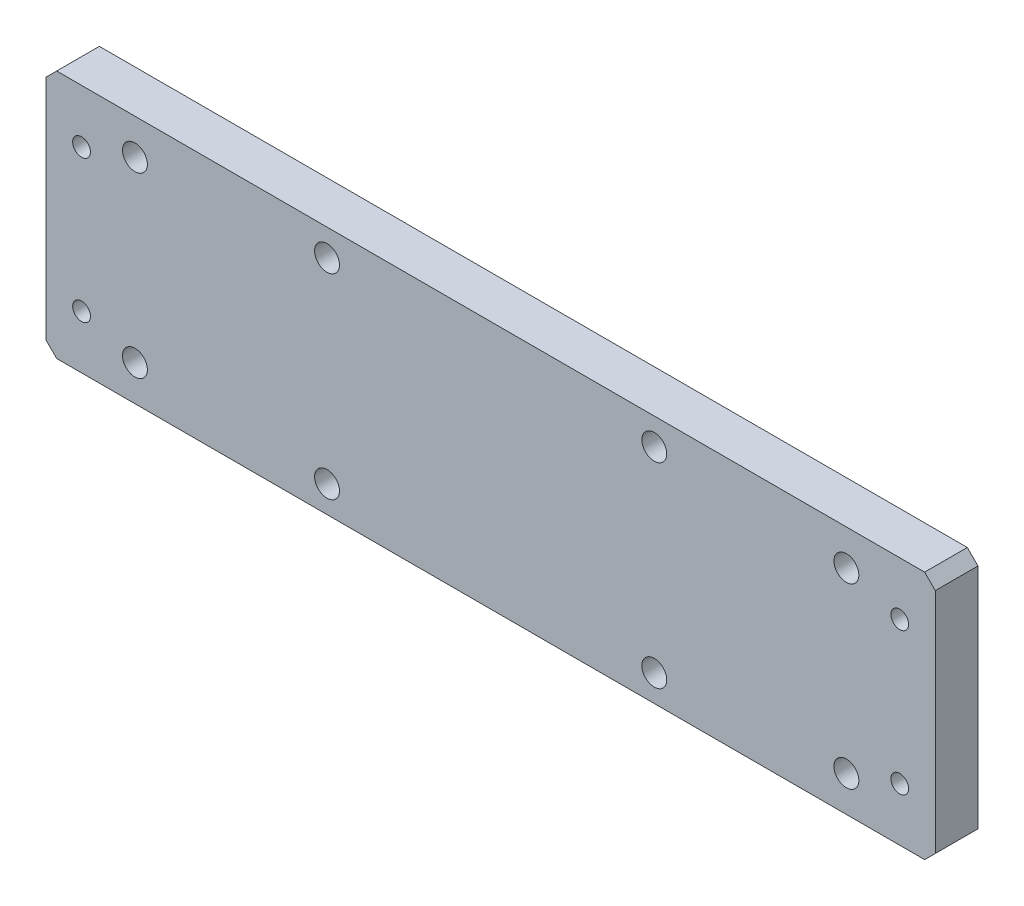
SolidWorks part; units mm, degrees
ref_plane "前视" through (0, 0, 0) normal (0, 0, 1) x (1, 0, 0)
ref_plane "上视" through (0, 0, 0) normal (0, 1, 0) x (1, 0, 0)
ref_plane "右视" through (0, 0, 0) normal (1, 0, 0) x (0, 0, -1)
sketch "草图1" plane through (0, 0, 0) normal (0, 0, 1) x (1, 0, 0)
  line L1 (-125, 35) -> (125, 35)
  line L2 (-125, 35) -> (-125, -35)
  line L3 (-125, -35) -> (125, -35)
  line L4 (125, 35) -> (125, -35)
  line L5 (-125, 35) -> (125, -35) construction
  line L6 (-125, -35) -> (125, 35) construction
  point P0 (0, 0)
  dimension "D1" = 70
  dimension "D2" = 250
extrude "凸台-拉伸1" add sketch "草图1" along normal blind 12
chamfer "倒角1" distance 3 angle 45 4 edges at (125, -35, 6) (125, 35, 6) (-125, -35, 6) (-125, 35, 6)
hole_wizard "Ø7.0 (7) 直径孔1" positions "草图3" profile "草图2" hole size "Ø7.0" standard "ISO" end condition through all
sketch "草图3" plane through (0, 0, 0) normal (0, 0, -1) x (-1, 0, 0)
  line L0 (0, 0) -> (0, 35) construction
  line L1 (-122, 35) -> (122, 35) construction
  line L3 (100, -25) -> (100, 25) construction
  line L6 (100, 0) -> (0, 0) construction
  line L8 (125, 32) -> (125, -32) construction
  point P0 (100, -25)
  point P2 (100, 25)
  point P14 (-100, 25)
  point P15 (-100, -25)
  dimension "D1" = 25
  dimension "D2" = 50
sketch "草图2" plane through (-100, -25, 0) normal (1, 0, 0) x (0, 1, 0)
  line L0 (0, 0) -> (0, 12)
  line L1 (0, 12) -> (3.5, 12)
  line L2 (3.5, 12) -> (3.5, 0)
  line L5 (3.5, 0) -> (0, 0)
  line L11 (0, -6.35) -> (0, 107.95) construction
  dimension "通孔孔直径" = 7
  dimension "通孔孔深度" = 12
hole_wizard "M6 螺纹孔1" positions "草图5" profile "草图4" tap size "M6" standard "GB" end condition through all
sketch "草图5" plane through (0, 0, 0) normal (0, 0, -1) x (-1, 0, 0)
  line L4 (115, 20) -> (115, -20) construction
  line L7 (0, 0) -> (0, -35) construction
  line L8 (122, -35) -> (-122, -35) construction
  line L10 (115, 0) -> (0, 0) construction
  line L12 (125, 32) -> (125, -32) construction
  point P26 (115, -20)
  point P28 (115, 20)
  point P55 (-115, 20)
  point P56 (-115, -20)
  dimension "D1" = 40
  dimension "D2" = 10
sketch "草图4" plane through (-115, -20, 0) normal (1, 0, 0) x (0, 1, 0)
  line L0 (0, 0) -> (0, 12)
  line L1 (0, 12) -> (2.5, 12)
  line L2 (2.5, 12) -> (2.5, 0)
  line L5 (2.5, 0) -> (0, 0)
  line L11 (0, -6.35) -> (0, 107.95) construction
  dimension "通孔螺纹孔钻头直径" = 5
  dimension "通孔螺纹孔钻头深度" = 12
cosmetic thread "孔螺蚊线1" parameters "D2"=6
cosmetic thread "孔螺蚊线2" parameters "D2"=6
cosmetic thread "孔螺蚊线3" parameters "D2"=6
cosmetic thread "孔螺蚊线4" parameters "D2"=6
hole_wizard "Ø7.0 (7) 直径孔2" positions "草图7" profile "草图6" hole size "Ø7.0" standard "ISO" end condition through all
sketch "草图7" plane through (0, 0, 0) normal (0, 0, -1) x (-1, 0, 0)
  point P0 (46, 27.5)
  point P3 (46, -27.5)
  point P6 (-46, 27.5)
  point P9 (-46, -27.5)
sketch "草图6" plane through (-46, 27.5, 0) normal (1, 0, 0) x (0, 1, 0)
  line L0 (0, 0) -> (0, 12)
  line L1 (0, 12) -> (3.5, 12)
  line L2 (3.5, 12) -> (3.5, 0)
  line L5 (3.5, 0) -> (0, 0)
  line L11 (0, -6.35) -> (0, 107.95) construction
  dimension "通孔孔直径" = 7
  dimension "通孔孔深度" = 12
